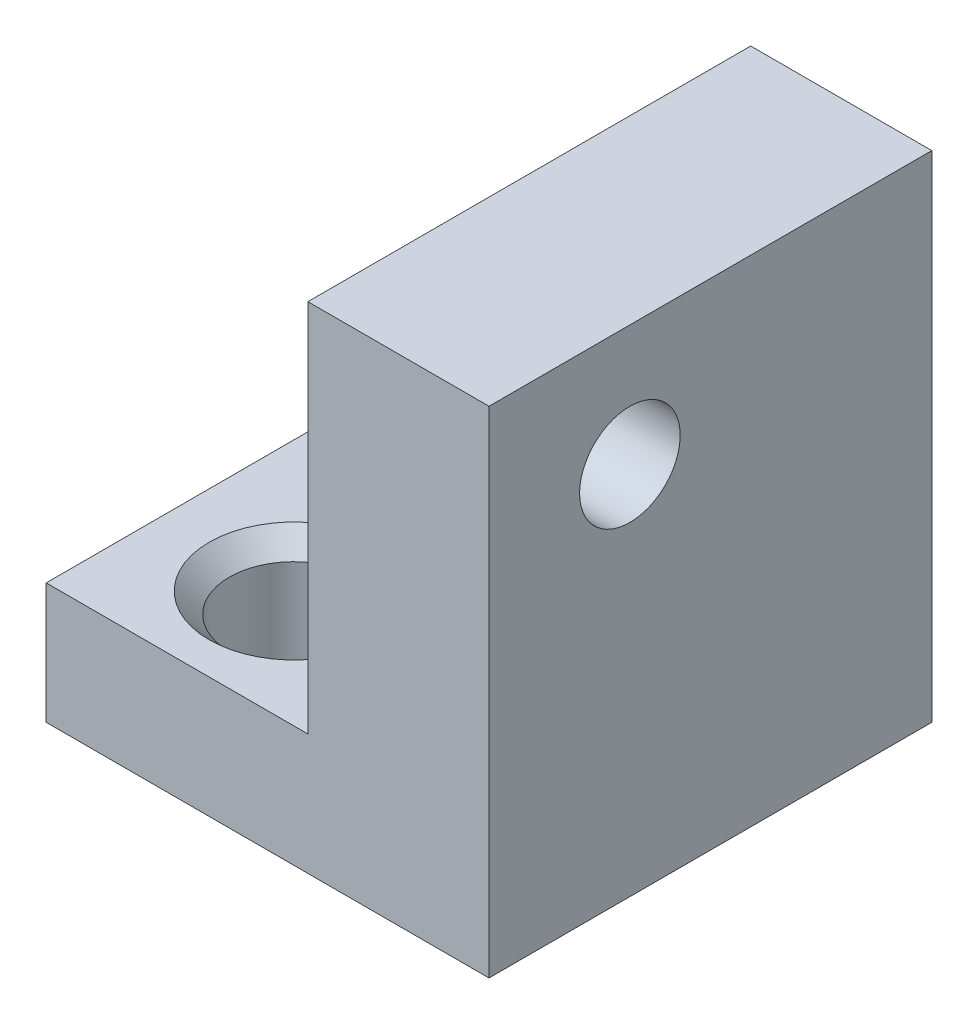
from build123d import *

# Parameters (mm, degrees)
SKETCH1_W             = 11
SKETCH1_H             = 11
BOSS_EXTRUDE1_DEPTH   = 3
SKETCH2_W             = 4.5
SKETCH2_H             = 11
BOSS_EXTRUDE2_DEPTH   = 9.3
M3_TAPPED_HOLE1_D     = 2.5
M3_TAPPED_HOLE1_DEPTH = 8.5
M3_TAPPED_HOLE1_TIP   = 0.751075774
SKETCH5_R             = 1.6
CUT_EXTRUDE1_DEPTH    = 13.123943253
CHAMFER1_SIZE         = 0.5


with BuildPart() as part:
    # Sketch1 → Boss-Extrude1 (new body)
    with BuildSketch(Plane(origin=(0, 0, 0), x_dir=(1, 0, 0), z_dir=(0, 1, 0))):
        Rectangle(SKETCH1_W, SKETCH1_H)
    extrude(amount=BOSS_EXTRUDE1_DEPTH)

    # Sketch2 → Boss-Extrude2 (add)
    with BuildSketch(Plane(origin=(0, 3, 0), x_dir=(1, 0, 0), z_dir=(0, 1, 0))):
        with Locations((3.25, 0)):
            Rectangle(SKETCH2_W, SKETCH2_H)
    extrude(amount=BOSS_EXTRUDE2_DEPTH)

    # M3 Tapped Hole1
    with Locations(Plane.ZY.offset(-1)):
        with Locations((2, 9.3)):
            Hole(M3_TAPPED_HOLE1_D / 2, depth=M3_TAPPED_HOLE1_DEPTH)
            with Locations((0, 0, -(M3_TAPPED_HOLE1_DEPTH + M3_TAPPED_HOLE1_TIP / 2))):  # 118° drill point
                Cone(0, M3_TAPPED_HOLE1_D / 2, M3_TAPPED_HOLE1_TIP, mode=Mode.SUBTRACT)

    # Sketch5 → Cut-Extrude1 (cut, through all)
    with BuildSketch(Plane(origin=(0, 3, 0), x_dir=(1, 0, 0), z_dir=(0, 1, 0))):
        with Locations(Location((-2.25, 2.6, 0), (0, 0, 270))):
            Circle(SKETCH5_R)
        with Locations(Location((-2.25, -2.6, 0), (0, 0, 270))):
            Circle(SKETCH5_R)
    extrude(amount=-CUT_EXTRUDE1_DEPTH, mode=Mode.SUBTRACT)

    # Chamfer1
    chamfer1_edges = [part.edges().sort_by_distance(p)[0] for p in [
        (-2.25, 3, -4.2),
        (-2.25, 3, 1),
    ]]
    chamfer(chamfer1_edges, length=CHAMFER1_SIZE)


solid = part.part
